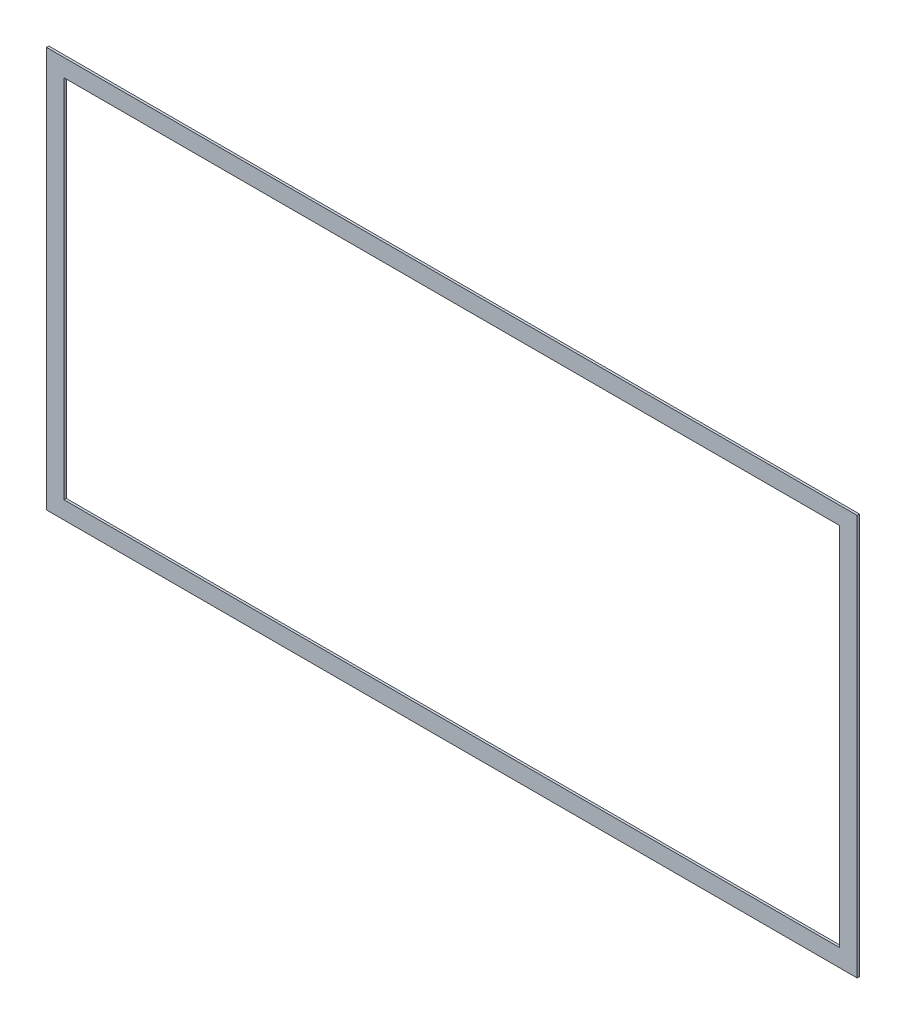
SolidWorks part; units mm, degrees
material "标准件"
ref_plane "前视基准面" through (0, 0, 0) normal (0, 0, 1) x (1, 0, 0)
ref_plane "上视基准面" through (0, 0, 0) normal (0, 1, 0) x (1, 0, 0)
ref_plane "右视基准面" through (0, 0, 0) normal (1, 0, 0) x (0, 0, -1)
sketch "草图1" plane through (0, 0, 0) normal (0, 0, 1) x (1, 0, 0)
  line L0 (-331, 156) -> (331, 156)
  line L1 (-346, -171) -> (346, -171)
  line L2 (-346, -171) -> (-346, 171)
  line L3 (-346, 171) -> (346, 171)
  line L4 (346, -171) -> (346, 171)
  line L5 (-346, -171) -> (346, 171) construction
  line L6 (-346, 171) -> (346, -171) construction
  line L7 (331, -156) -> (331, 156)
  line L8 (-331, -156) -> (331, -156)
  line L9 (-331, -156) -> (-331, 156)
  point P0 (0, 0)
  dimension "D1" = 692
  dimension "D2" = 342
  dimension "D3" = 15
extrude "凸台-拉伸1" add sketch "草图1" along normal mid plane 2
